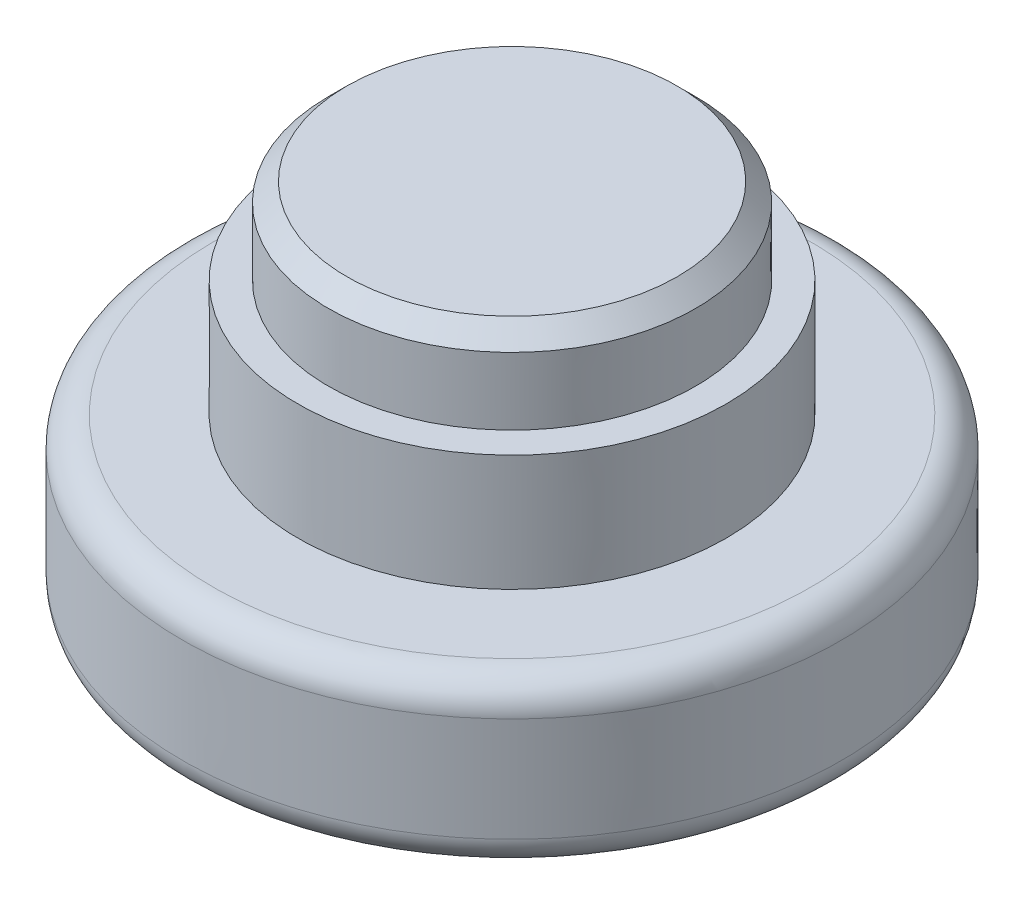
SolidWorks part; units mm, degrees
material "1023 碳钢板 (SS)"
ref_plane "Front Plane" through (0, 0, 0) normal (0, 0, 1) x (1, 0, 0)
ref_plane "Top Plane" through (0, 0, 0) normal (0, 1, 0) x (1, 0, 0)
ref_plane "Right Plane" through (0, 0, 0) normal (1, 0, 0) x (0, 0, -1)
sketch "Sketch1" plane through (0, 0, 0) normal (0, 0, 1) x (1, 0, 0)
  line L0 (0, 0) -> (27, 0)
  line L1 (27, 0) -> (30, -3)
  line L2 (0, 0) -> (0.0017, -64.4758)
  line L3 (30, -3) -> (30, -14)
  line L4 (30, -14) -> (35, -14)
  line L5 (35, -14) -> (35, -33)
  line L6 (35, -33) -> (48.85, -33)
  line L7 (40.3311, -63.527) -> (50.5909, -59.7164)
  line L8 (53.85, -55.0292) -> (53.85, -38)
  line L9 (0.0017, -64.4758) -> (34.8444, -64.4758)
  line L10 (34.8444, -64.4758) -> (34.8444, -63.527)
  line L11 (40.3311, -63.527) -> (34.8444, -63.527)
  arc A0 (53.85, -38) -> (48.85, -33) centre (48.85, -38) ccw
  arc A1 (50.5909, -59.7164) -> (53.85, -55.0292) centre (48.85, -55.0292) ccw
  point P0 (30, 0)
  dimension "D1" = 3
  dimension "D2" = 3
revolve "Revolve1" add sketch "Sketch1" angle 360 about L2
